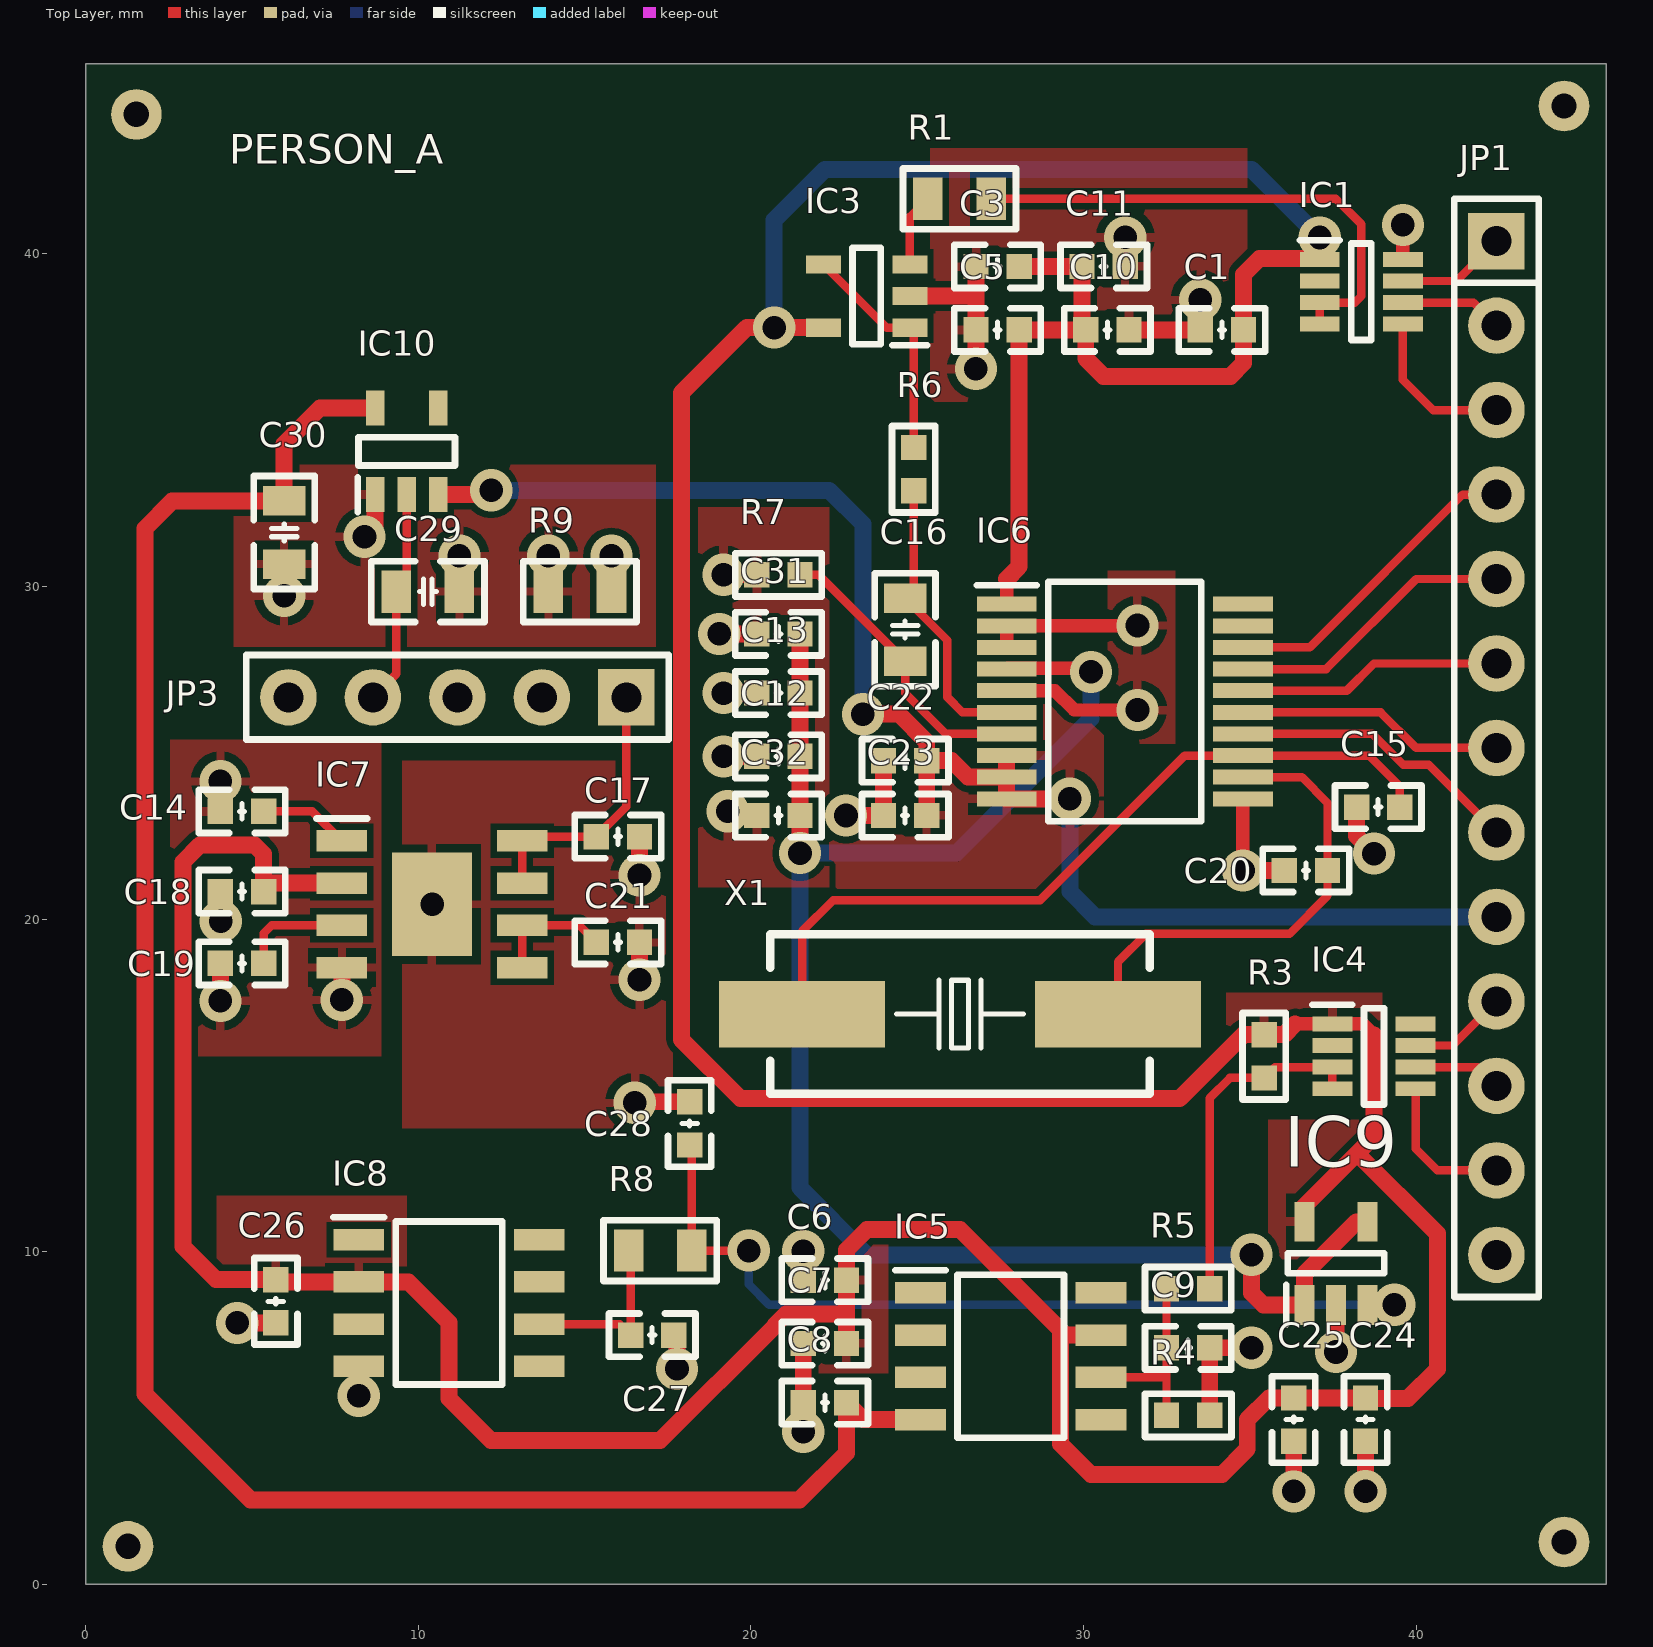
[diagram p0: Top Layer view]
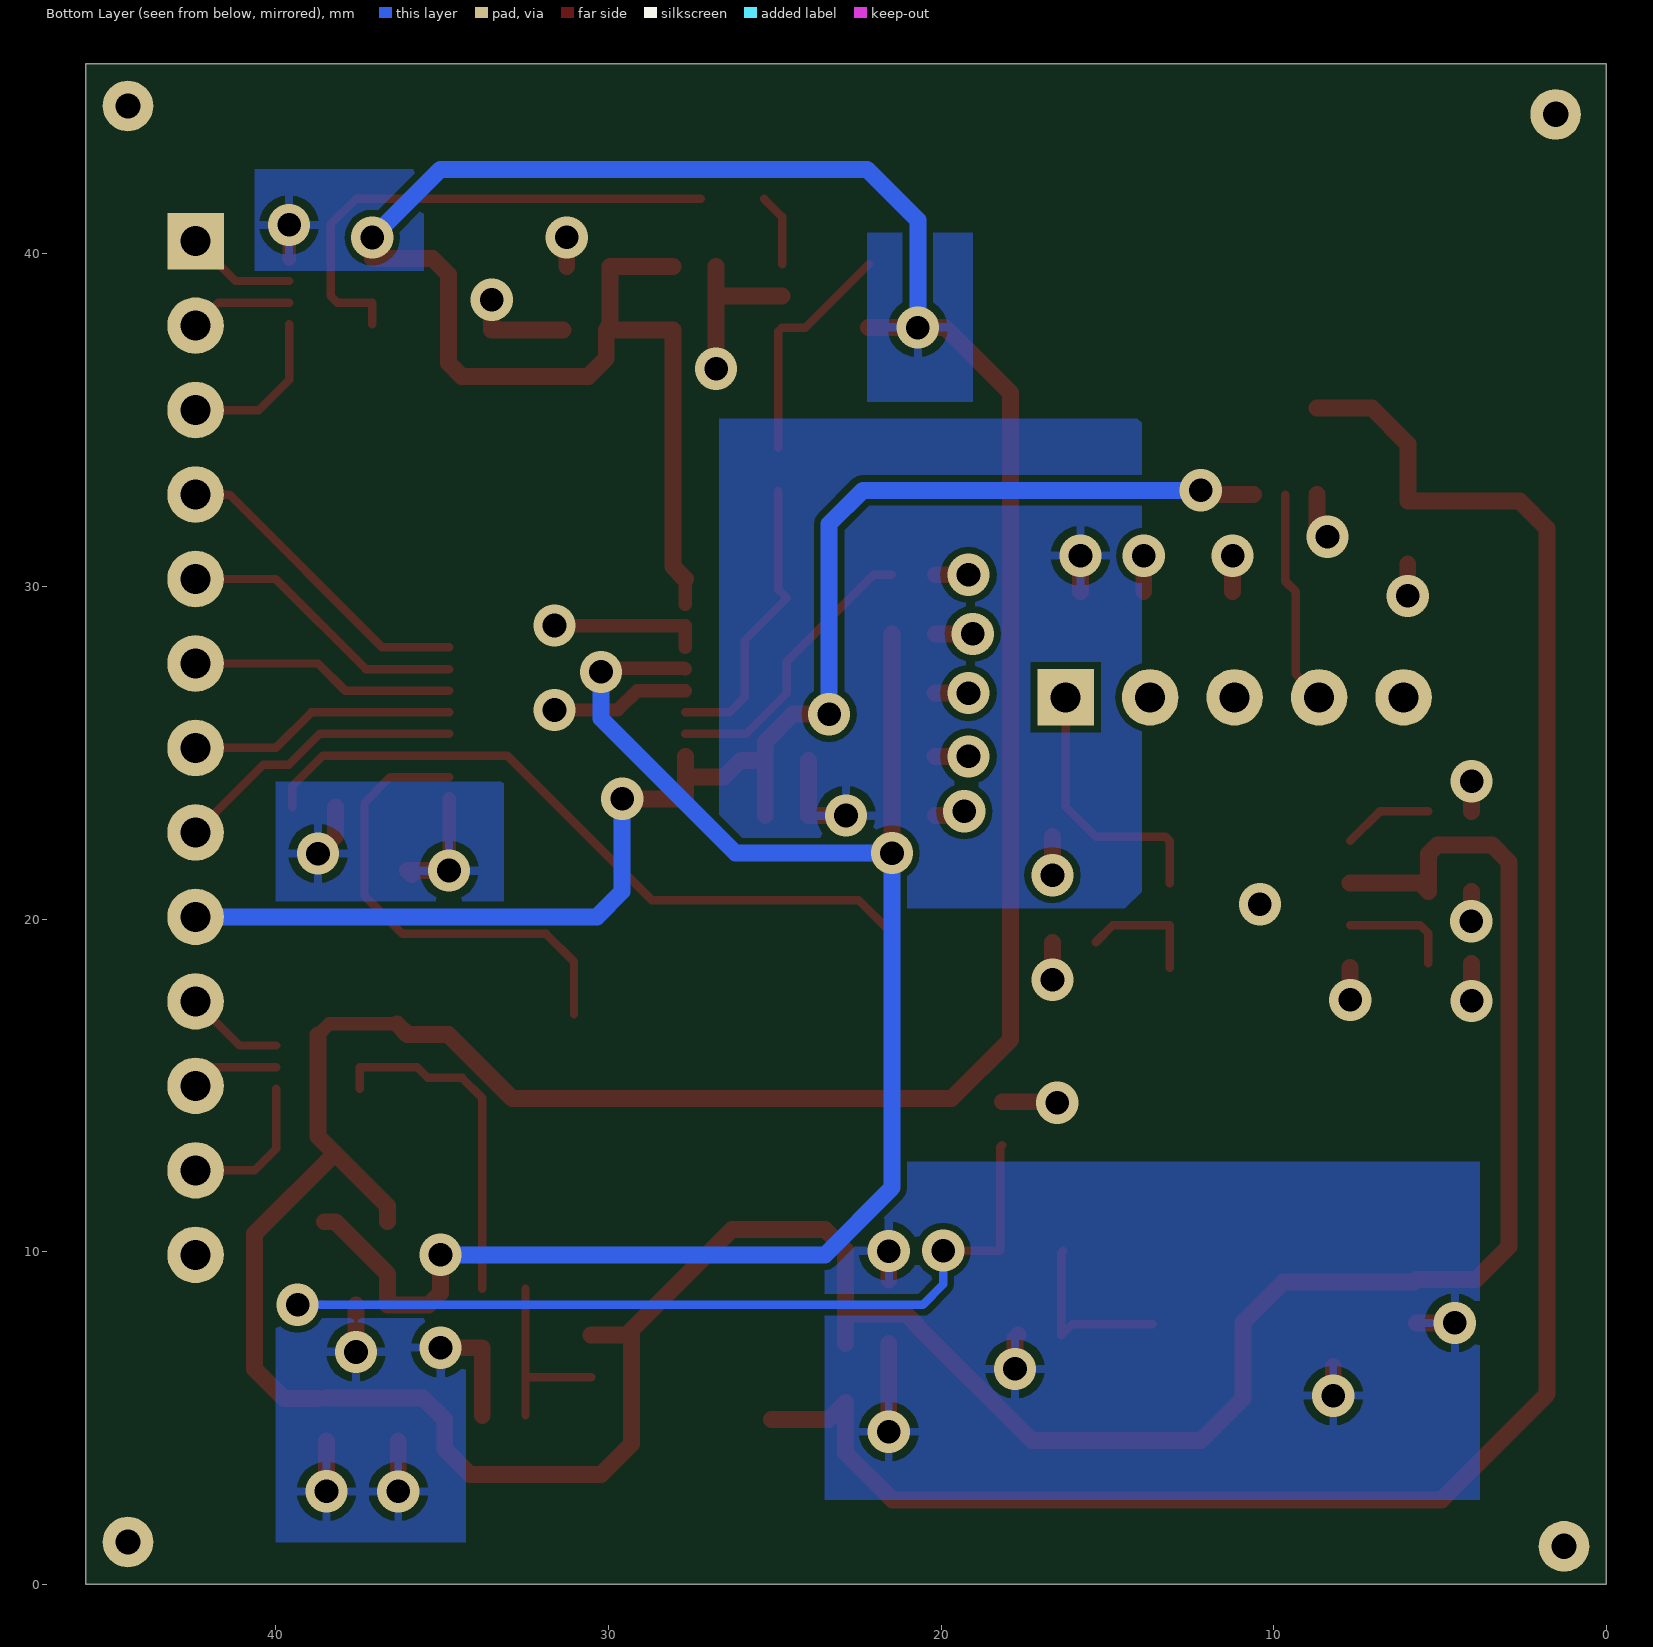
[diagram p1: Bottom Layer view, seen from below]
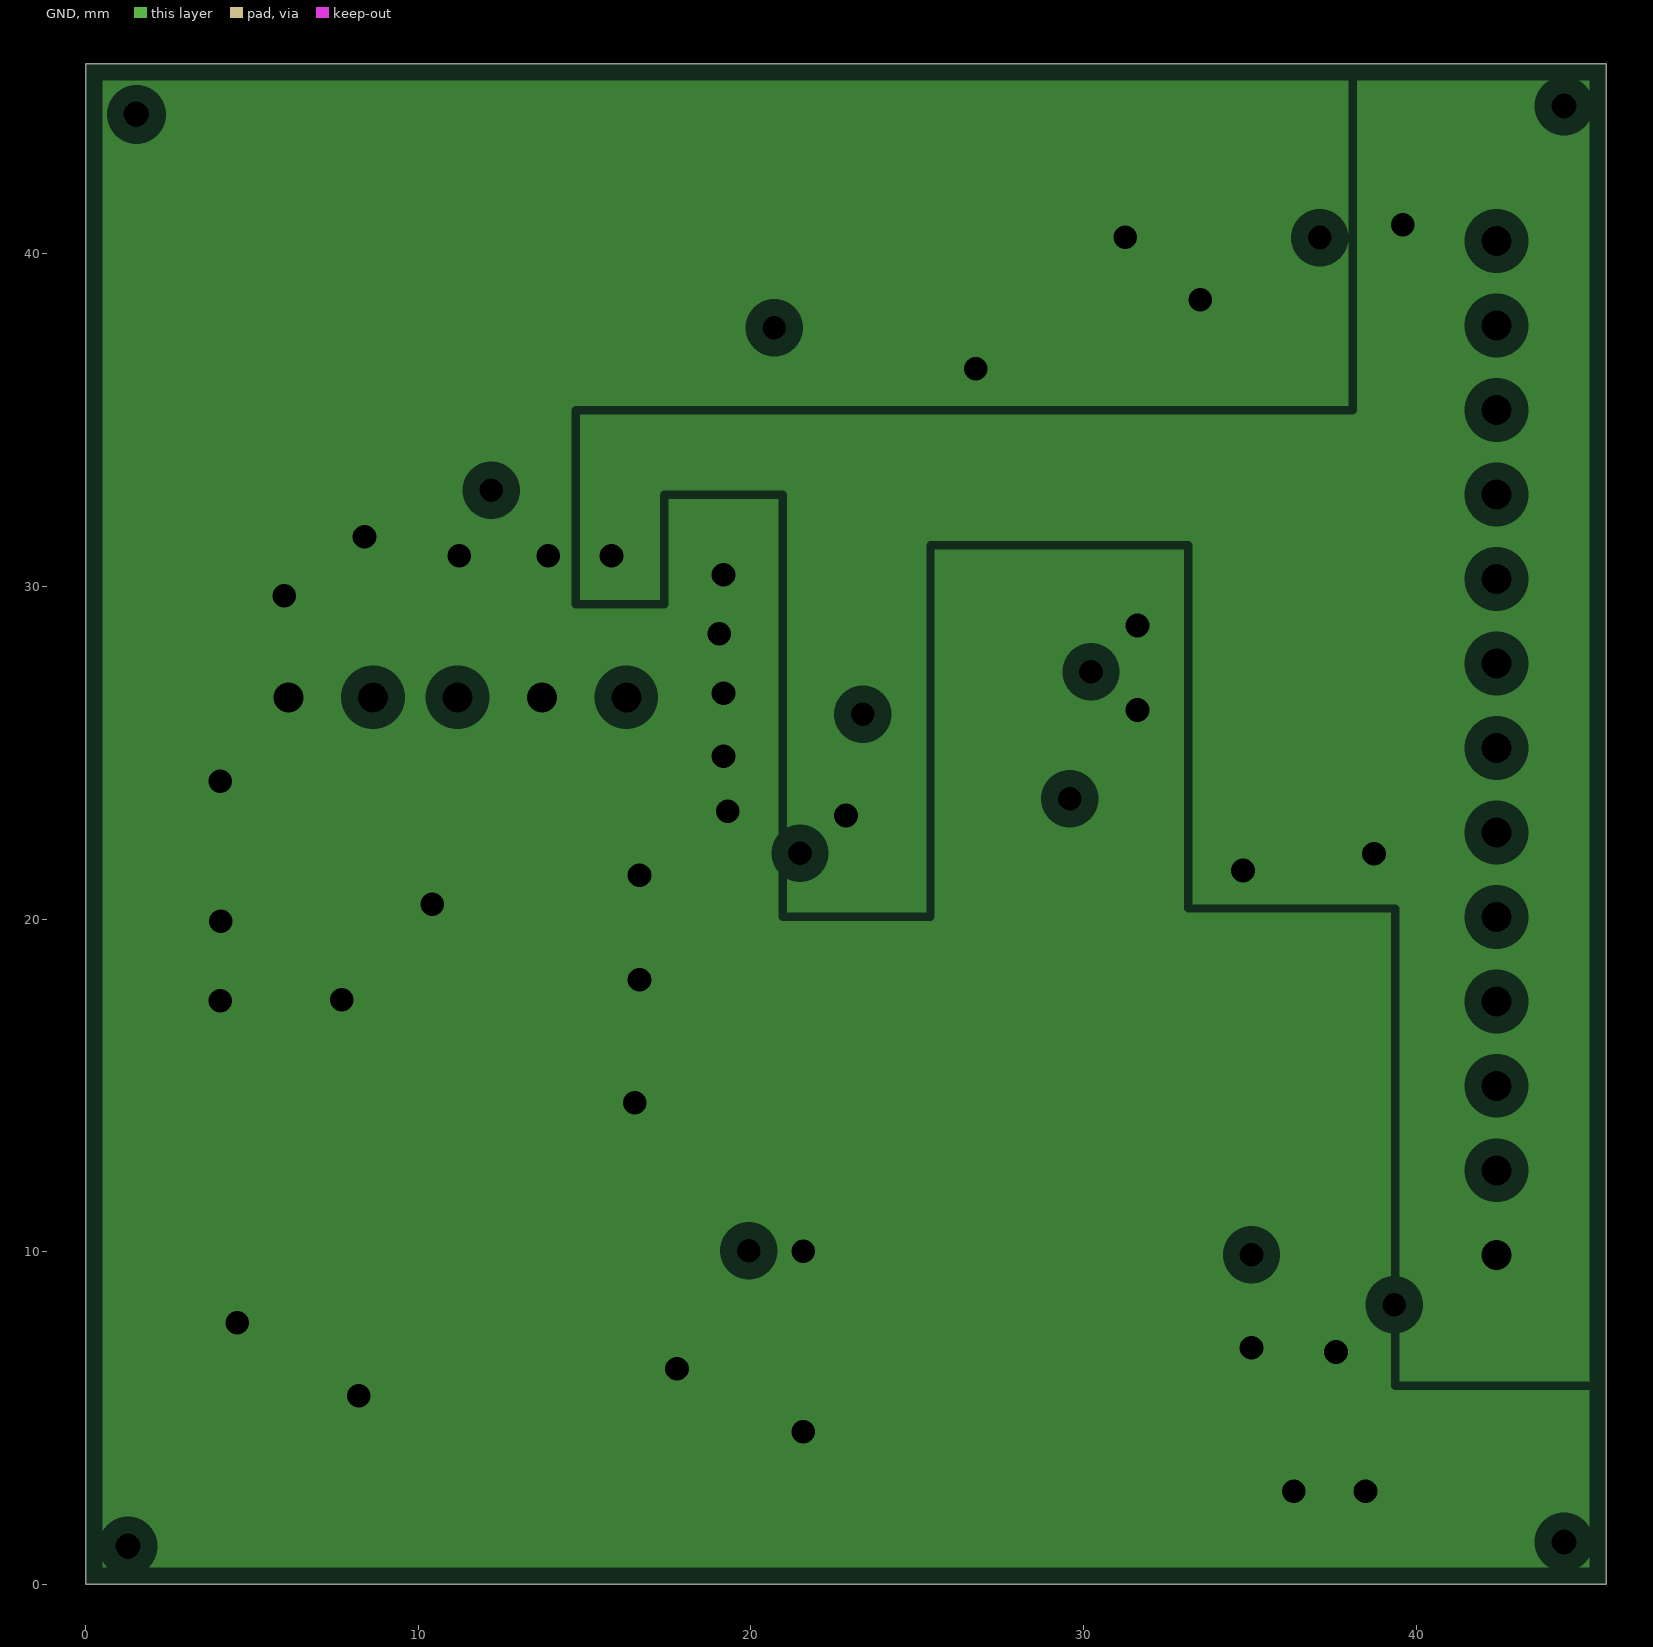
[diagram p2: GND, clearances drawn from the general rule]
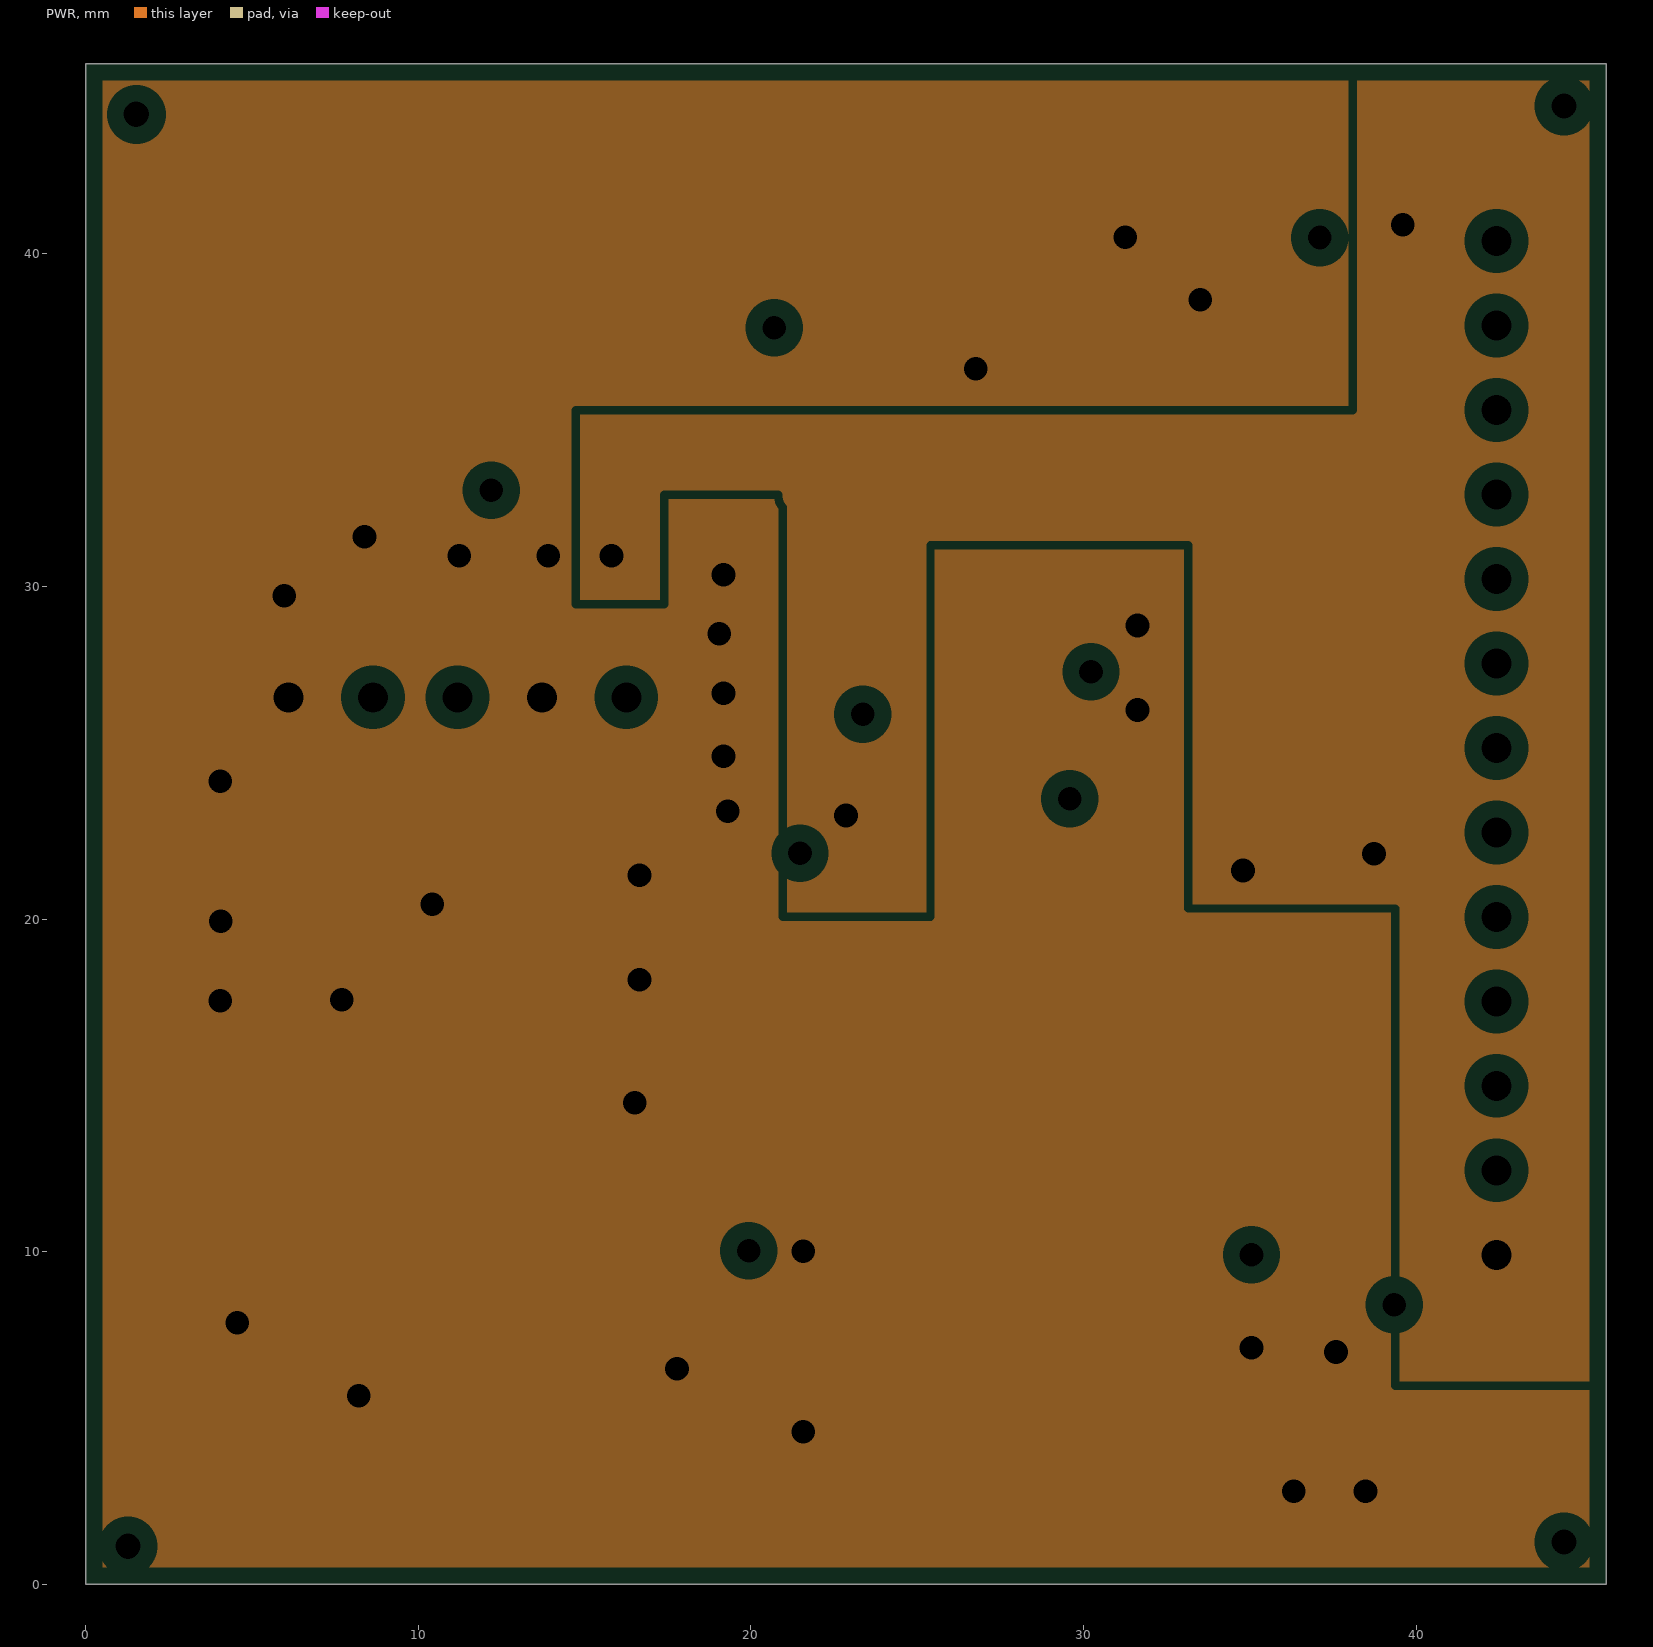
[diagram p3: PWR, clearances drawn from the general rule]
# Altium PCB MISC82306.PcbDoc
Units mm, origin at the board's own origin, x right, y up, seen from the top; angles counter-clockwise.
Board outline 45.72 x 45.72 mm, 4 copper layers (Top Layer, GND, PWR, Bottom Layer), stack 0.778 mm thick; 50 components, 33 nets, 176 pads, 46 vias.

## Layer stack, top to bottom
Top Solder: solder mask 0.0102, Solder Resist, Dk 3.5
Top Layer: signal copper 0.0356
Dielectric 1: core 0.254, FR-4, Dk 4.2
GND: plane copper 0.036, net AGND
Dielectric 3: prepreg 0.127, Dk 4.2
PWR: plane copper 0.036, net AGND
Dielectric 2: core 0.254, Dk 4.2
Bottom Layer: signal copper 0.0356
Bottom Solder: solder mask 0.0102, Solder Resist, Dk 3.5

## Board outline
0,0 45.72,0 45.72,45.72 0,45.72

## Design rules (kind name [scope] priority, off if disabled: settings)
Clearance [All] p1: gap=0.2 except(0.254: Arc-Arc)
HoleToHoleClearance [All] p1: gap=0.508 allowstackedmicrovias=TRUE
MinimumSolderMaskSliver [All] p1: minsoldermaskwidth=0
PlaneClearance [All] p1: clearance=0.508
PlaneConnect [All] p1: planeconnectstyle=Relief reliefexpansion=0.508 reliefentries=4 reliefconductorwidth=0.254 reliefairgap=0.254
PolygonConnect [All] p1: connectstyle=Relief reliefconductorwidth=0.254 reliefentries=4 polygonreliefangle="90 Angle" airgapwidth=0.254
RoutingVias [All] p1: holewidth=0.711 width=1.27 viastyle="Through Hole" minholewidth=0.711 minwidth=1.27 maxholewidth=0.711 maxwidth=1.27
SilkToSilkClearance [All] p1: silktosilkclearance=0
SilkToSolderMaskClearance [IsPad] p1: minsilkscreentomaskgap=0 clearancetoexposedcopper=TRUE
SolderMaskExpansion [All] p1: expansion=0.102
Width PWR [InNetClass('PWR')] p1: maxlimit=0.51 minlimit=0.4 preferedwidth=0.508 minimp=50.000000 maximp=50.000000 favimp=50.000000
Width Width_1 [All] p2: maxlimit=0.51 minlimit=0.254 preferedwidth=0.254
24 further rules are at their usual default settings.

## Classes and differential pairs
net class PWR: A+5V AGND D-5V DGND REF+2V5

## Components (designator, comment, footprint, x,y, rotation, side; value= is the part's Value field where it differs from the comment)
C1 "0.1uF" "C 0603_L" 34.163,37.719 r180 top
C3 "100nF" "C 0603_L" 27.417,39.624 r180 top
C5 "1uF" "C 0603_L" 27.417,37.719 r180 top
C6 "0.1uF" "C 0603_L" 22.225,9.144 r180 top
C7 "0.1uF" "C 0603_L" 22.225,7.239 r180 top
C8 "0.1uF" "C 0603_L" 22.225,5.461 r0 top
C9 "0.1uF" "C 0603_L" 33.147,7.112 r0 top
C10 "1uF" "C 0603_L" 30.719,37.719 r0 top
C11 "100nF" "C 0603_L" 30.607,39.624 r0 top
C12 "1uF" "C 0603_L" 20.828,24.892 r180 top
C13 "100nF" "C 0603_L" 20.828,26.797 r180 top
C14 "10uF" "C 0603_L" 4.699,23.241 r180 top
C15 "20pF" "C 0603_L" 38.862,23.368 r180 top
C16 "220pF" "C 0805_L" 24.638,28.702 r90 top
C17 "10uF" "C 0603_L" 16.002,22.479 r0 top
C18 "10uF" "C 0603_L" 4.699,20.828 r180 top
C19 "1uF" "C 0603_L" 4.699,18.669 r180 top
C20 "20pF" "C 0603_L" 36.688,21.463 r180 top
C21 "1uF" "C 0603_L" 16.002,19.304 r0 top
C22 "100nF" "C 0603_L" 24.638,24.765 r180 top
C23 "1uF" "C 0603_L" 24.638,23.114 r180 top
C24 "1uF" "C 0603_L" 38.481,4.953 r270 top
C25 "100nF" "C 0603_L" 36.322,4.953 r270 top
C26 "100nF" "C 0603_L" 5.715,8.509 r270 top
C27 "100nF" "C 0603_L" 17.033,7.493 r0 top
C28 "100nF" "C 0603_L" 18.161,13.858 r90 top
C29 "2.2uF" "C 0805_L" 10.287,29.845 r180 top
C30 "2.2uF" "C 0805_L" 5.969,31.623 r270 top
C31 "10uF" "C 0603_L" 20.828,28.575 r0 top
C32 "100nF" "C 0603_L" 20.828,23.114 r0 top
IC1 "AD5660ARJZ-2500RL7" SOT65P280X145-8N 38.354,38.862 r0 top
IC3 "OPA387DBVT" SOT95P280X100-5N 23.48,38.735 r180 top
IC4 "AD5660ARJZ-2500RL7" SOT65P280X145-8N 38.735,15.875 r0 top
IC5 "AD820ARZ" SOIC127P600X175-8N 27.813,6.858 r0 top
IC6 "ADS1255IDBR" SOP65P780X200-20N 31.242,26.543 r0 top
IC7 "ADM7150ARDZ-5.0-R7" SOIC127P600X175-9N 10.414,20.447 r0 top
IC8 "ADR4525ARZ" SOIC127P600X175-8N 10.922,8.458 r0 top
IC9 "OPA387DBVT" SOT95P280X145-5N 37.592,9.652 r90 top
IC10 "ADP7182AUJZ-5.0-R7" SOT95P280X100-5N 9.652,34.066 r90 top
JP1 "HDR-1X13" HDR2.54-LI-13P 42.418,25.146 r270 top
JP3 "HDR-1X5" HDR2.54-LI-5P 11.176,26.67 r180 top
R1 "50R" "R 0805_L" 26.274,41.656 r180 top
R3 "10K" "R 0603_L" 35.433,15.875 r90 top
R4 "1K" "R 0603_L" 33.147,5.08 r180 top
R5 "10K" "R 0603_L" 33.147,8.89 r0 top
R6 "10R" "R 0603_L" 24.892,33.528 r270 top
R7 "10R" "R 0603_L" 20.828,30.353 r0 top
R8 "10K" "R 0805_L" 17.272,10.033 r0 top
R9 "0R" "R 0805_L" 14.859,29.845 r0 top
X1 "7.68MHz" "OSC HC-49SMD" 26.289,17.145 r180 top

## Footprints (in the part's own frame and the unit in brackets; to place one, negate y for a bottom-side part, rotate by r counter-clockwise, add the part's x,y. Pads: shape width x height; smd on the part's side, far side on the other; paste and mask are expansions set on the pad)
"C 0603_L" [mil] "无极性贴片电容"
  rect 30x30 smd: 1(-25.59,0) 2(25.59,0)
  silkscreen extent -51,-26 51,26, body extent -31,-16 31,16, height 32
"C 0805_L" [mil] "无极性贴片电容"
  rect 35x50 smd: 1(-37.4,0) 2(37.4,0)
  silkscreen extent -67,-36 67,36, body extent -39,-24 39,24, height 20
HDR2.54-LI-5P [mm] "排针，5脚"
  rect 1.7x1.7 hole 0.9: 1(-5.08,0)
  round 1.7 hole 0.9: 2(-2.54,0) 3(0,0) 4(2.54,0) 5(5.08,0)
  silkscreen extent -6.35,-1.27 6.35,1.27, body extent -6.35,-1.27 6.35,1.27, height 8.5
HDR2.54-LI-13P [mm] "排针，13脚"
  rect 1.7x1.7 hole 0.9: 1(-15.24,0)
  round 1.7 hole 0.9: 2(-12.7,0) 3(-10.16,0) 4(-7.62,0) 5(-5.08,0) 6(-2.54,0) 7(0,0) 8(2.54,0) 9(5.08,0) 10(7.62,0) 11(10.16,0) 12(12.7,0) 13(15.24,0)
  silkscreen extent -16.51,-1.27 16.51,1.27, body extent -16.51,-1.27 16.51,1.27, height 8.5
"OSC HC-49SMD" [mm]
  rect 5x2 smd: 1(-4.75,0) 2(4.75,0)
  silkscreen extent -5.7,-2.4 5.7,2.4, body extent -6.5,-2.32 6.5,2.33, height 4.63
"R 0603_L" [mil] "1/10W贴片电阻"
  rect 30x30 smd: 1(-25.59,0) 2(25.59,0)
  silkscreen extent -51,-26 51,26, body extent -31,-16 32,16, height 16
"R 0805_L" [mil] "1/8W贴片电阻"
  rect 35x50 smd: 1(-37.4,0) 2(37.4,0)
  silkscreen extent -67,-36 67,36, body extent -39,-25 39,25, height 20
SOIC127P600X175-8N [mm]
  rect 1.525x0.65 smd: 1(-2.712,1.905) 2(-2.712,0.635) 3(-2.712,-0.635) 4(-2.712,-1.905) 5(2.712,-1.905) 6(2.712,-0.635) 7(2.712,0.635) 8(2.712,1.905)
  silkscreen extent -3.47,-2.45 1.6,2.58, body extent -3,-2.45 3,2.45, height 1.75
SOIC127P600X175-9N [mm]
  rect 1.525x0.65 smd: 1(-2.712,1.905) 2(-2.712,0.635) 3(-2.712,-0.635) 4(-2.712,-1.905) 5(2.712,-1.905) 6(2.712,-0.635) 7(2.712,0.635) 8(2.712,1.905)
  rect 2.41x3.098 smd: 9(0,0)
  silkscreen extent -3.47,2.58 -1.95,2.58, body extent -3,-2.45 3,2.45, height 1.75
SOP65P780X200-20N [mm]
  rect 1.8x0.45 smd: 1(-3.55,2.925) 2(-3.55,2.275) 3(-3.55,1.625) 4(-3.55,0.975) 5(-3.55,0.325) 6(-3.55,-0.325) 7(-3.55,-0.975) 8(-3.55,-1.625) 9(-3.55,-2.275) 10(-3.55,-2.925) 11(3.55,-2.925) 12(3.55,-2.275) 13(3.55,-1.625) 14(3.55,-0.975) 15(3.55,-0.325) 16(3.55,0.325) 17(3.55,0.975) 18(3.55,1.625) 19(3.55,2.275) 20(3.55,2.925)
  silkscreen extent -4.45,-3.6 2.3,3.6, body extent -3.9,-3.6 3.9,3.6, height 1.9
SOT65P280X145-8N [mm]
  rect 1.2x0.45 smd: 1(-1.25,0.975) 2(-1.25,0.325) 3(-1.25,-0.325) 4(-1.25,-0.975) 5(1.25,-0.975) 6(1.25,-0.325) 7(1.25,0.325) 8(1.25,0.975)
  silkscreen extent -1.85,-1.45 0.3,1.55, body extent -1.4,-1.45 1.4,1.45, height 1.45
SOT95P280X100-5N [mm]
  rect 1.05x0.55 smd: 1(-1.3,0.95) 2(-1.3,0) 3(-1.3,-0.95) 4(1.3,-0.95) 5(1.3,0.95)
  silkscreen extent -1.83,-1.45 0.43,1.48, body extent -1.4,-1.45 1.4,1.45, height 1
SOT95P280X145-5N [mm]
  rect 1.2x0.6 smd: 1(-1.25,0.95) 2(-1.25,0) 3(-1.25,-0.95) 4(1.25,-0.95) 5(1.25,0.95)
  silkscreen extent -1.85,-1.45 0.3,1.5, body extent -1.4,-1.45 1.4,1.45, height 1.2

## Part data
C1 C3 C5 C6 C7 C8 C9 C10 C11 C12 C13 C14 C15 C16 C17 C18 C19 C20 C21 C22 C23 C24 C25 C26 C27 C28 C29 C30 C31 C32: library part C, "Non-polar chip capacitor"
IC1: library part AD5620ARJZ-1500RL7, "Integrated Circuit"
IC3 IC4 IC5 IC6 IC7 IC8 IC9 IC10: "Integrated Circuit"
JP1: library part "Header 13", "13P connector"
JP3: library part "Header 5", "5P connector"
R1 R3 R5: library part R, "PTFR0603B100RN9"
R4 R6 R7 R8 R9: library part R, "Chip resistor"
X1: library part XTAL-2P, "2-pin passive crystal oscillator"

## Free pads (board coordinates)
  round 1.524 hole 0.762: 2(1.524,44.196) 3(1.27,1.143) 4(44.45,44.45) 5(44.45,1.27)

## Via types
v1: diameter 1.27, hole 0.71, Top Layer to Bottom Layer, 46 vias

## Nets (pads, with @x,y where several pads share a name; then routed paths per layer and width w, separated by ;. In a path a pad name is that pad's centre, name@x,y a point inside that pad or via, vN(x,y) a via of type N, cw(c..) or ccw(c..) an arc to the next point about the centre after c; other vN are vias at no path point)
A+5V: C1.1 C3.1 C5.1 C6.1 C7.1 C10.1 C11.1 C18.1 C24.1 C25.1 C26.1 IC1.1 IC3.5 IC4.1 IC5.7 IC6.1 IC7.2 IC8.2 IC9.5 R3.2 | length 180.2
  Top Layer w0.4: IC6.1 27.692,30.22 ; 36.363,16.85 IC4.1 38.395,16.85 38.735,16.51 ; IC1.1 37.104,39.867 v1(37.104,40.493)
  Top Layer w0.508: IC7.2 5.603,21.082 C18.1 5.349,21.956 5.08,22.225 3.429,22.225 2.921,21.717 2.921,10.16 3.922,9.159 C26.1 5.781,9.093 IC8.2 9.703,9.093 10.922,7.874 10.922,5.588 12.192,4.318 17.272,4.318 20.74,7.786 20.74,7.808 21.06,8.128 22.875,8.128 ; C7.1 22.875,8.128 ; IC5.7 29.464,7.493 29.309,7.648 ; C24.1 C25.1 35.575,5.603 34.925,4.953 34.925,4.064 34.163,3.302 30.226,3.302 29.309,4.219 29.309,7.648 ; 22.875,8.128 C6.1 22.875,10.048 23.495,10.668 26.289,10.668 29.309,7.648
  Top Layer w0.51: IC3.5 v1(20.701,37.785) 19.878,37.785 17.907,35.814 17.907,16.383 19.685,14.605 32.893,14.605 34.813,16.525 R3.2 36.038,16.525 36.363,16.85 ; 27.692,30.22 28.067,30.595 C5.1 C10.1 ; C3.1 C11.1 29.957,37.831 C10.1 ; IC9.5 36.642,11.369 38.227,12.954 ; IC1.1@37.104,39.867 35.295,39.867 34.813,39.385 C1.1 34.813,36.718 34.417,36.322 30.607,36.322 30.069,36.86 C10.1 ; 38.735,16.51 38.735,13.462 38.227,12.954 ; C24.1@38.75,5.588 39.751,5.588 40.64,6.477 40.64,10.541 38.227,12.954
  Bottom Layer w0.51: v1(20.701,37.785) 20.701,41.021 22.225,42.545 35.052,42.545 v1(37.104,40.493)
AGND: C1.2 C3.2 C5.2 C6.2 C7.2 C8.1 C9.2 C10.2 C11.2 C12.2 C13.2 C14.2 C17.2 C18.2 C19.2 C21.2 C24.2 C25.2 C26.2 C27.2 C28.2 C29.1 C30.2 C31.1 C32.1 IC3.2 IC6.2 IC6.3 IC6.5 IC7.4 IC7.9 IC8.4 IC9.2 IC10.1 JP3.2 JP3.5 R4.1 R7.1 R9.1 | length 48.3
  Top Layer w0.4: IC6.5 29.139,26.868 29.718,26.289 v1(31.623,26.289) ; IC6.3 IC6.2 31.104,28.818 v1@31.115,28.829
  Top Layer w0.508: v1(4.049,17.541) C19.2 ; v1@4.049,20.178 C18.2 ; C14.2 v1(4.049,24.145) ; v1(4.557,7.859) C26.2 ; v1(5.969,29.718) C30.2 ; v1(7.702,17.571) IC7.4 ; v1(8.21,5.67) IC8.4 ; v1@8.702,31.816 IC10.1 ; C29.1 v1(11.237,30.922) ; R9.1 v1(13.909,30.927) ; v1@16.413,14.508 C28.2 ; v1(16.652,18.176) C21.2 ; v1(16.652,21.321) C17.2 ; C27.2 17.78,7.396 v1(17.78,6.477) ; v1@19.05,23.114 C32.1 ; v1(19.05,28.575) C31.1 ; v1(19.177,24.892) C12.2 ; v1(19.177,26.797) C13.2 ; v1(19.177,30.353) R7.1 ; v1(21.575,4.587) C8.1 C7.2 ; C6.2 v1(21.575,10.018) ; IC3.2 26.767,38.735 ; v1(26.767,36.546) C5.2 26.767,38.735 ; C3.2 26.767,38.735 ; C11.2 v1(31.257,40.498) ; C10.2 C1.2 v1(33.513,38.623) ; R4.1 C9.2 v1(35.052,7.112) ; v1(36.322,2.794) C25.2 ; v1@37.592,7.239 IC9.2 ; v1(38.481,2.794) C24.2
  other v1: 37.592,6.985 16.51,14.478 4.064,19.939 10.414,20.447 19.304,23.241 31.623,28.829 8.382,31.496
D+3V3: C22.1 C23.1 IC6.8 IC6.9 IC6.10 IC10.3 JP1.9 | length 45.1
  Top Layer w0.51: IC10.3 12.065,32.766 v1(12.192,32.893) ; v1(23.368,26.162) 24.45,26.162 25.288,25.324 C22.1 ; C23.1 C22.1 ; IC6.8@27.692,24.888 IC6.9 ; v1(29.591,23.622) 29.587,23.618 IC6.10 IC6.9 ; C22.1 26.035,24.765 26.532,24.268 IC6.9
  Bottom Layer w0.51: v1(12.192,32.893) 22.352,32.893 23.368,31.877 v1(23.368,26.162) ; v1(29.591,23.622) 29.591,20.828 30.353,20.066 JP1.9
D-5V: C8.2 C30.1 IC5.4 IC10.5 | length 62.4
  Top Layer w0.51: IC10.5 7.045,35.366 5.969,34.29 C30.1 2.601,32.573 1.778,31.75 1.778,5.715 4.953,2.54 21.463,2.54 22.875,3.952 C8.2 23.383,4.953 IC5.4
DGND: C15.2 C20.2 C22.2 C23.2 IC1.8 IC6.11 JP1.13 R9.2 | length 10.2
  Top Layer w0.4: v1@34.671,21.59 34.792,21.711 IC6.11 ; IC1.8 v1(39.604,40.874)
  Top Layer w0.51: R9.2 v1(15.809,30.927) ; v1(22.86,23.114) C23.2 C22.2 ; v1@34.671,21.59 v1(34.798,21.463) C20.2 C20.2@35.911,21.336 ; C15.2 38.212,22.494 v1(38.735,21.971)
DIN1: IC1.7 JP1.1 | length 3.3
  Top Layer w0.254: IC1.7 41.219,39.187 JP1.1
DIN2: IC4.7 JP1.10 | length 3
  Top Layer w0.254: IC4.7 41.092,16.2 JP1.10
JD: IC3.3 R1.2 | length 2.2
  Top Layer w0.254: IC3.3 24.78,41.112 R1.2
NetC9_1: C9.1 IC5.6 R4.2 R5.1 | length 5.8
  Top Layer w0.254: IC5.6 32.497,6.223 ; R4.2 32.497,6.223 ; R5.1 32.497,6.223
NetC14_1: C14.1 IC7.1 | length 2.7
  Top Layer w0.254: C14.1 6.813,23.241 IC7.1
NetC15_1: C15.1 IC6.13 X1.2 | length 23.7
  Top Layer w0.254: X1.2 21.539,19.634 22.479,20.574 28.702,20.574 33.046,24.918 IC6.13 38.582,24.918 39.512,23.988 C15.1
NetC16_1: C16.1 IC6.7 R7.2 | length 8.8
  Top Layer w0.254: R7.2 22.037,30.353 C16.1 24.638,26.797 25.867,25.568 IC6.7
NetC16_2: C16.2 IC6.6 R6.2 | length 8.8
  Top Layer w0.254: R6.2 24.892,29.906 C16.2 25.908,28.382 25.908,26.67 26.36,26.218 IC6.6
NetC17_1: C17.1 IC7.7 IC7.8 JP3.1 | length 8.1
  Top Layer w0.254: IC7.7 IC7.8 13.253,22.479 C17.1 16.256,23.383 JP3.1
NetC19_1: C19.1 IC7.3 | length 3.4
  Top Layer w0.254: C19.1 5.349,19.573 5.588,19.812 IC7.3
NetC20_1: C20.1 IC6.12 X1.1 | length 14.4
  Top Layer w0.254: X1.1 31.039,18.72 31.877,19.558 36.195,19.558 37.338,20.701 C20.1 37.338,23.495 36.565,24.268 IC6.12
NetC21_1: C21.1 IC7.5 IC7.6 | length 3.7
  Top Layer w0.254: IC7.5 IC7.6 14.844,19.812 C21.1
NetC27_1: C27.1 IC8.6 R8.1 | length 5.5
  Top Layer w0.254: IC8.6 16.053,7.823 C27.1 16.383,9.972 R8.1
NetC28_1: C28.1 IC9.3 R8.2 | length 26.4
  Top Layer w0.254: C28.1 18.222,13.147 R8.2 v1(19.939,10.033) ; IC9.3 v1(39.35,8.402)
  Bottom Layer w0.254: v1(19.939,10.033) 19.939,9.017 20.554,8.402 v1(39.35,8.402)
NetC29_2: C29.2 IC10.2 JP3.4 | length 6.5
  Top Layer w0.254: JP3.4 9.337,27.371 C29.2 9.652,30.16 IC10.2
NetIC1_3: IC1.3 IC1.4 R1.1 | length 15.6
  Top Layer w0.254: R1.1 37.592,41.656 38.354,40.894 38.354,38.735 38.156,38.537 IC1.3 IC1.4
NetIC3_1: IC3.1 IC3.4 R6.1 | length 7
  Top Layer w0.254: IC3.4 24.08,37.785 IC3.1 24.892,37.673 R6.1
NetIC4_3: IC4.3 IC4.4 R3.1 R5.2 | length 10.5
  Top Layer w0.254: R5.2 33.797,14.62 34.402,15.225 R3.1 35.758,15.55 IC4.3 IC4.4
NetIC6_14: IC6.14 JP1.8 | length 8.9
  Top Layer w0.254: IC6.14 38.687,25.568 39.617,24.638 40.386,24.638 JP1.8
NetIC6_15: IC6.15 JP1.7 | length 8.1
  Top Layer w0.254: IC6.15 38.933,26.218 40.005,25.146 JP1.7
NetIC6_16: IC6.16 JP1.6 | length 8
  Top Layer w0.254: IC6.16 37.917,26.868 38.735,27.686 JP1.6
NetIC6_17: IC6.17 JP1.5 | length 8.7
  Top Layer w0.254: IC6.17 37.297,27.518 40.005,30.226 JP1.5
NetIC6_18: IC6.18 JP1.4 | length 9.5
  Top Layer w0.254: IC6.18 36.804,28.168 41.402,32.766 JP1.4
REF+2V5: C12.1 C13.1 C31.2 C32.2 IC6.4 IC9.1 IC9.4 | length 51.8
  Top Layer w0.4: IC6.4 27.717,27.543 30.115,27.543 v1(30.226,27.432)
  Top Layer w0.508: v1(21.478,21.986) C32.2 C31.2 ; v1(35.052,9.906) 35.052,8.763 35.413,8.402 IC9.1 36.642,9.337 38.207,10.902 IC9.4
  Bottom Layer w0.508: v1(30.226,27.432) 30.226,26.035 26.177,21.986 v1(21.478,21.986) 21.478,11.923 23.495,9.906 v1(35.052,9.906)
SCLK1: IC1.6 JP1.2 | length 3.1
  Top Layer w0.254: IC1.6 41.727,38.537 JP1.2
SCLK2: IC4.6 JP1.11 | length 2.7
  Top Layer w0.254: IC4.6 41.854,15.55 JP1.11
SYNC1: IC1.5 JP1.3 | length 4.9
  Top Layer w0.254: IC1.5 39.604,36.215 40.513,35.306 JP1.3
SYNC2: IC4.5 JP1.12 | length 4.5
  Top Layer w0.254: IC4.5 39.985,13.101 40.64,12.446 JP1.12
pads on no net: IC1.2 IC4.2 IC4.8 IC5.1 IC5.2 IC5.3 IC5.5 IC5.8 IC6.19 IC6.20 IC8.1 IC8.3 IC8.5 IC8.7 IC8.8 IC10.4 JP3.3

## Polygon pours and split planes (outlines as drawn)
D+3V3 on Top Layer "D" (solid, remove dead copper, pour order 126): 30.607,19.685 30.607,25.527 28.756,27.378 22.352,27.378 22.352,19.685
AGND on Top Layer "G" (solid, remove dead copper, pour order 124): 30.734,30.48 32.766,30.48 32.766,25.273 30.734,25.273
AGND on Top Layer "G" (solid, remove dead copper, pour order 122): 25.4,43.18 34.925,43.18 34.925,35.56 25.527,35.56 25.4,35.687
A+5V on Top Layer "G" (solid, remove dead copper, pour order 120): 19.685,11.43 23.622,11.43 24.13,11.43 24.13,6.35 19.685,6.35
A+5V on Top Layer "G" (solid, remove dead copper, pour order 116): 35.56,13.97 39.751,13.97 39.751,9.779 35.56,9.779
A+5V on Top Layer "G" (solid, remove dead copper, pour order 114): 34.29,17.78 38.989,17.78 38.989,16.256 34.29,16.256
A+5V on Top Layer "G" (solid, remove dead copper, pour order 110): 3.937,11.684 9.652,11.684 9.652,7.747 3.937,7.747
AGND on Top Layer "G" (solid, remove dead copper, pour order 108): 9.525,24.765 17.526,24.765 17.653,24.638 17.653,13.716 9.525,13.716
AGND on Top Layer "G" (solid, remove dead copper, pour order 106): 2.54,25.4 8.89,25.4 8.89,15.875 2.54,15.875
AGND on Top Layer "G" (solid, remove dead copper, pour order 104): 4.445,33.655 17.145,33.655 17.145,28.194 4.445,28.194
AGND on Top Layer "G" (solid, remove dead copper, pour order 102): 18.415,32.385 22.352,32.385 22.352,20.955 18.415,20.955
A+5V on Bottom Layer "D" (solid, remove dead copper, pour order 138): 19.05,40.64 22.225,40.64 22.225,35.56 19.05,35.56
DGND on Bottom Layer "D" (solid, remove dead copper, pour order 136): 13.97,34.925 14.097,35.052 26.67,35.052 26.67,20.32 14.478,20.32 13.97,20.828
AGND on Bottom Layer "D" (solid, remove dead copper, pour order 134): 34.29,8.001 40.132,8.001 40.005,7.874 40.005,1.27 34.29,1.27
AGND on Bottom Layer "D" (solid, remove dead copper, pour order 132): 3.81,12.7 23.495,12.7 23.495,2.54 3.81,2.54
DGND on Bottom Layer "D" (solid, remove dead copper, pour order 130): 35.56,42.545 40.64,42.545 40.64,39.497 35.56,39.497
DGND on Bottom Layer "D" (solid, remove dead copper, pour order 128): 40.005,19.05 40.005,24.13 33.274,24.13 33.147,24.257 33.147,19.05
DGND on GND (split plane): 45.21,6.098 39.499,6.098 39.499,20.32 39.49,20.37 39.462,20.412 39.42,20.44 39.37,20.449 33.276,20.449 33.276,20.828 33.276,28.702 33.276,31.242 33.267,31.292 33.239,31.334 33.197,31.362 33.147,31.371 25.4,31.371 25.35,31.362 25.308,31.334 25.28,31.292 25.271,31.242 25.271,28.956 25.271,20.195 21.084,20.195 21.084,21.336 21.084,25.908 21.084,32.766 21.075,32.816 21.047,32.858 21.005,32.886 20.955,32.895 17.399,32.895 17.349,32.886 17.307,32.858 17.279,32.816 17.27,32.766 17.27,32.258 17.27,29.593 14.861,29.593 14.861,34.29 14.861,35.177 38.1,35.177 38.15,35.186 38.192,35.214 38.22,35.256 38.229,35.306 38.229,41.275 38.229,45.21 45.21,45.21
AGND on GND (split plane): 37.971,41.275 37.971,35.435 14.732,35.435 14.682,35.426 14.64,35.398 14.612,35.356 14.603,35.306 14.603,34.29 14.603,34.036 14.603,29.464 14.612,29.414 14.64,29.372 14.682,29.344 14.732,29.335 17.399,29.335 17.449,29.344 17.491,29.372 17.519,29.414 17.528,29.464 17.528,32.258 17.528,32.637 20.826,32.637 20.826,25.908 20.826,21.336 20.826,20.066 20.835,20.016 20.863,19.974 20.905,19.946 20.955,19.937 25.4,19.937 25.45,19.946 25.492,19.974 25.52,20.016 25.529,20.066 25.529,28.956 25.529,31.113 33.018,31.113 33.018,28.702 33.018,20.828 33.018,20.32 33.027,20.27 33.055,20.228 33.097,20.2 33.147,20.191 39.241,20.191 39.241,5.969 39.25,5.919 39.278,5.877 39.32,5.849 39.37,5.84 45.21,5.84 45.21,0.51 0.51,0.51 0.51,45.21 37.971,45.21
DGND on PWR (split plane): 45.21,6.098 39.499,6.098 39.499,20.32 39.49,20.37 39.462,20.412 39.42,20.44 39.37,20.449 33.276,20.449 33.276,31.242 33.267,31.292 33.239,31.334 33.197,31.362 33.147,31.371 25.4,31.371 25.35,31.362 25.308,31.334 25.28,31.292 25.271,31.242 25.271,21.463 25.271,20.195 21.084,20.195 21.084,31.75 21.084,32.385 21.075,32.435 21.047,32.477 21.043,32.479 21.008,32.522 20.979,32.575 20.962,32.632 20.957,32.687 20.957,32.692 20.957,32.766 20.948,32.816 20.92,32.858 20.878,32.886 20.828,32.895 17.399,32.895 17.349,32.886 17.307,32.858 17.279,32.816 17.27,32.766 17.27,29.593 14.861,29.593 14.861,35.177 38.1,35.177 38.15,35.186 38.192,35.214 38.22,35.256 38.229,35.306 38.229,45.21 45.21,45.21
AGND on PWR (split plane): 37.971,35.435 14.732,35.435 14.682,35.426 14.64,35.398 14.612,35.356 14.603,35.306 14.603,29.464 14.612,29.414 14.64,29.372 14.682,29.344 14.732,29.335 17.399,29.335 17.449,29.344 17.491,29.372 17.519,29.414 17.528,29.464 17.528,32.637 20.704,32.637 20.706,32.604 20.727,32.518 20.761,32.436 20.807,32.361 20.826,32.339 20.826,31.75 20.826,20.066 20.835,20.016 20.863,19.974 20.905,19.946 20.955,19.937 25.4,19.937 25.45,19.946 25.492,19.974 25.52,20.016 25.529,20.066 25.529,21.463 25.529,31.113 33.018,31.113 33.018,20.32 33.027,20.27 33.055,20.228 33.097,20.2 33.147,20.191 39.241,20.191 39.241,5.969 39.25,5.919 39.278,5.877 39.32,5.849 39.37,5.84 45.21,5.84 45.21,0.51 0.51,0.51 0.51,45.21 37.971,45.21

## Other copper
GND (plane layer: these items are gaps in the copper):
  lines w0.254: 14.732,34.036 14.732,35.306 25.273,35.306 36.957,35.306 38.1,35.306 38.1,41.275 38.1,45.72 ; 14.732,34.29 14.732,29.464 17.018,29.464 ; 16.891,29.464 17.399,29.464 17.399,32.258 17.399,32.766 20.066,32.766 20.955,32.766 20.955,25.908 20.955,21.336 20.955,20.066 25.4,20.066 25.4,28.956 25.4,31.242 32.639,31.242 33.147,31.242 33.147,28.702 33.147,20.828 33.147,20.32 38.608,20.32 39.37,20.32 39.37,5.969 45.593,5.969
PWR (plane layer: these items are gaps in the copper):
  lines w0.254: 38.1,45.72 38.1,35.306 35.433,35.306 14.732,35.306 14.732,29.464 17.399,29.464 17.399,32.766 20.828,32.766 20.828,32.692 ccw(c21.262,32.692) 20.955,32.385 20.955,31.75 20.955,20.066 25.4,20.066 25.4,21.463 25.4,31.242 33.147,31.242 33.147,20.32 39.37,20.32 39.37,5.969 45.72,5.969

## Silkscreen, mask and mechanical layers (free items; w line width, h text height)
Top Overlay:
  text "PERSON_A" at 4.318,42.418 h1.52
Mechanical 1:
  the board outline again, w0.254